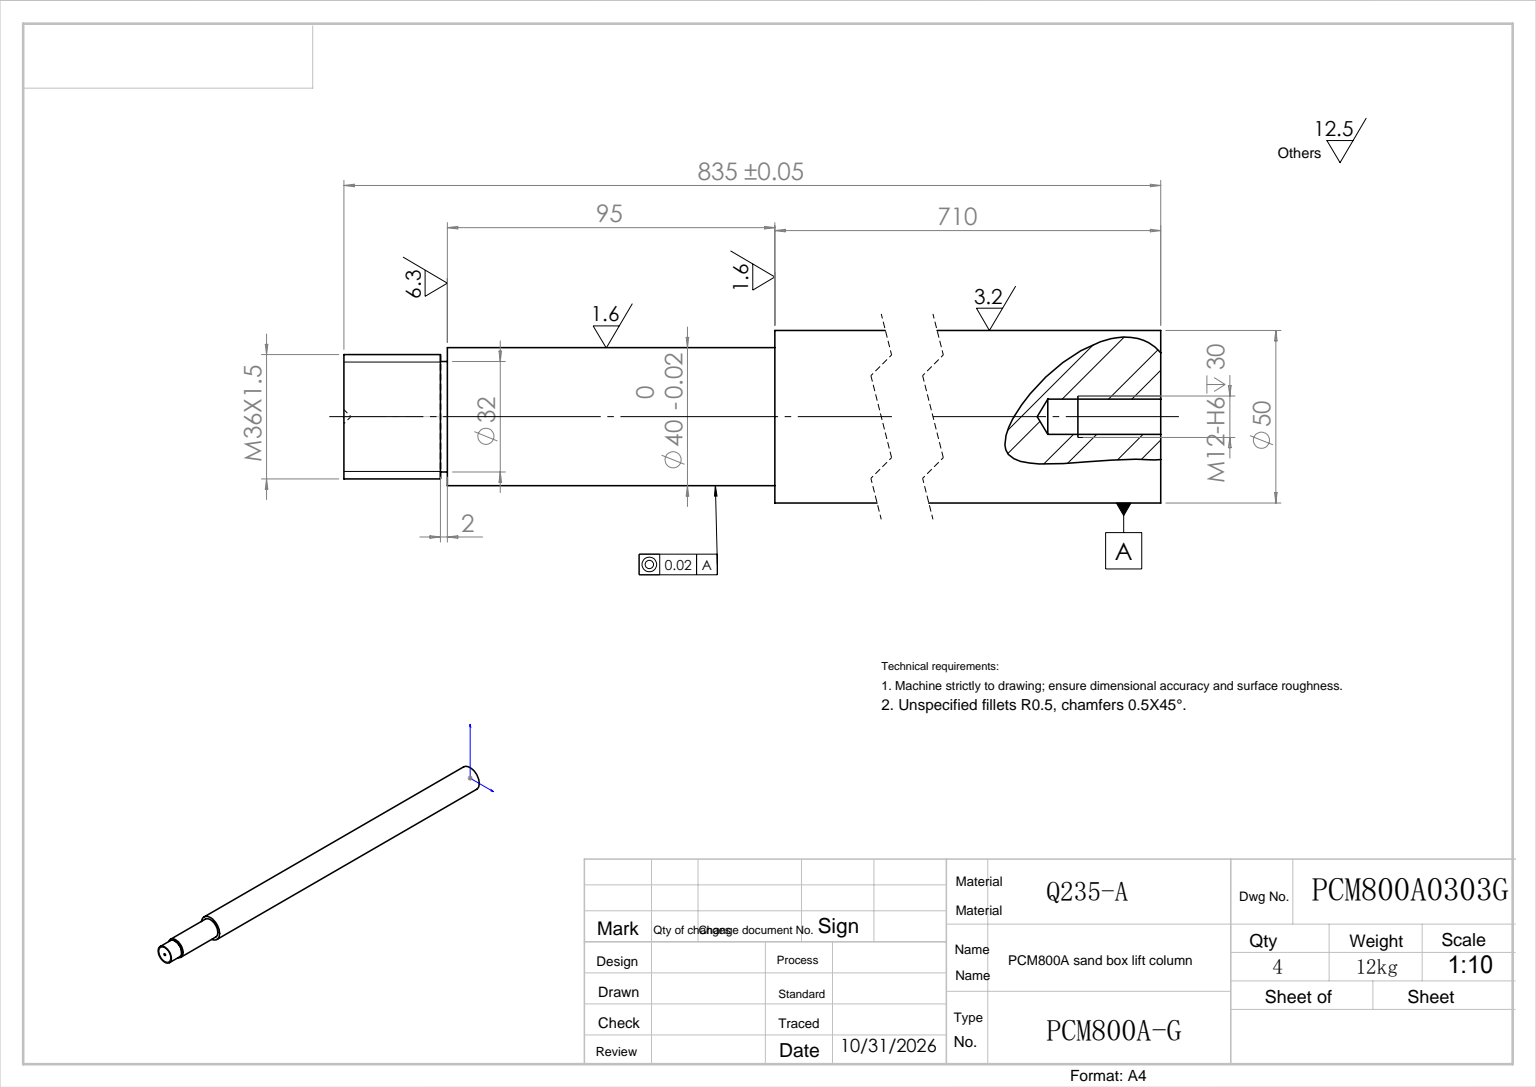
SolidWorks part; units mm, degrees
material "普通碳钢"
ref_plane "前视基准面" through (0, 0, 0) normal (0, 0, 1) x (1, 0, 0)
ref_plane "上视基准面" through (0, 0, 0) normal (0, 1, 0) x (1, 0, 0)
ref_plane "右视基准面" through (0, 0, 0) normal (1, 0, 0) x (0, 0, -1)
sketch "草图1" plane through (0, 0, 0) normal (0, 0, 1) x (1, 0, 0)
  circle A0 centre (0, 0) radius 25
extrude "拉伸1" add sketch "草图1" along normal blind 710
sketch "草图2" plane through (0, 0, 710) normal (0, 0, 1) x (1, 0, 0)
  circle A0 centre (0, 0) radius 20
extrude "拉伸2" add sketch "草图2" along normal blind 95
sketch "草图3" plane through (0, 0, 805) normal (0, 0, 1) x (1, 0, 0)
  circle A0 centre (0, 0) radius 18
extrude "拉伸3" add sketch "草图3" along normal blind 30
cosmetic thread "装饰螺纹线3" parameters "D1"=28, "D2"=31.67
hole_wizard "M12 螺纹孔1" positions "草图6" profile "草图5" tap size "M12" standard "GB"
sketch "草图6" plane through (0, 0, 0) normal (0, 0, -1) x (-1, 0, 0)
  point P0 (0, 0)
sketch "草图5" plane through (0, 0, 0) normal (1, 0, 0) x (0, 1, 0)
  line L0 (0, 0) -> (0, 35.8144)
  line L1 (0, 35.8144) -> (5.1, 32.75)
  line L2 (5.1, 32.75) -> (5.1, 0)
  line L5 (5.1, 0) -> (0, 0)
  line L10 (0, 35.8144) -> (-5.1, 32.75) construction
  line L11 (0, -6.35) -> (0, 107.95) construction
  dimension "螺纹孔钻头直径" = 10.2
  dimension "螺纹孔钻头深度" = 32.75
  dimension "导头角度" = 118
cosmetic thread "孔螺蚊线1" parameters "D1"=24, "D2"=12
sketch "草图7" plane through (0, 0, 0) normal (0, 1, 0) x (1, 0, 0)
  line L0 (0, -835) -> (0, -818.764) construction
  line L1 (-18, -835) -> (18, -835) construction
  line L2 (-2, -835) -> (0, -833)
  line L3 (-2, -835) -> (0, -835)
  line L4 (0, -835) -> (0, -833)
  dimension "D1" = 2
  dimension "D2" = 2
revolve "切除-旋转1" cut sketch "草图7" angle 360 about L0
sketch "草图8" plane through (0, 0, 805) normal (0, 0, 1) x (1, 0, 0)
  circle A0 centre (0, 0) radius 16
  circle A1 centre (0, 0) radius 20
  dimension "D1" = 32
  dimension "D2" = 40
extrude "切除-拉伸1" cut sketch "草图8" along normal blind 2
